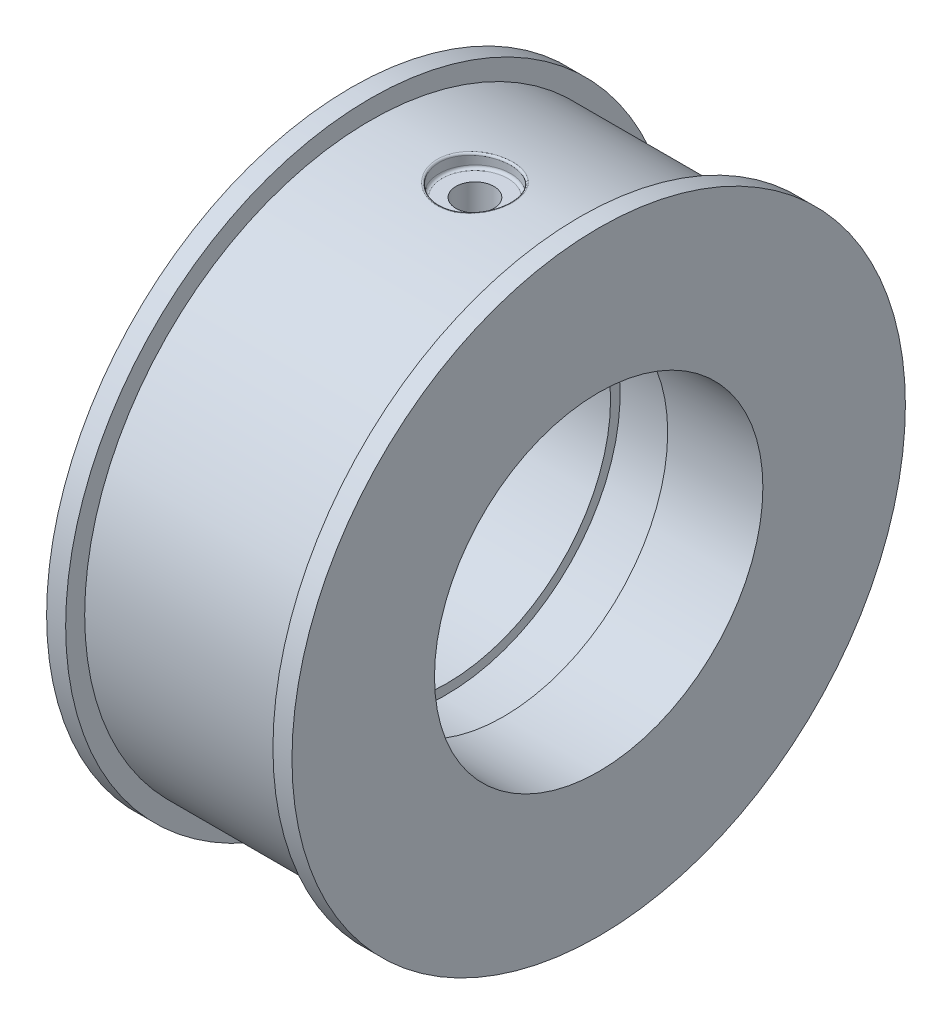
SolidWorks part; units mm, degrees
ref_plane "Front Plane" through (0, 0, 0) normal (0, 0, 1) x (1, 0, 0)
ref_plane "Top Plane" through (0, 0, 0) normal (0, 1, 0) x (1, 0, 0)
ref_plane "Right Plane" through (0, 0, 0) normal (1, 0, 0) x (0, 0, -1)
sketch "Sketch1" plane through (0, 0, 0) normal (0, 0, 1) x (1, 0, 0)
  line L0 (-19.0368, 0) -> (19.2228, 0) construction
  line L1 (-8.3897, 17.25) -> (-8.3897, 32)
  line L2 (-8.3897, 32) -> (-6.3897, 32)
  line L3 (-6.3897, 32) -> (-6.3897, 30)
  line L4 (-6.3897, 30) -> (15.6103, 30)
  line L5 (15.6103, 30) -> (15.6103, 32.223)
  line L6 (15.6103, 32.223) -> (17.6103, 32.223)
  line L7 (17.6103, 32.223) -> (17.6103, 17.25)
  line L8 (17.6103, 17.25) -> (7.6103, 17.25)
  line L9 (7.6103, 17.25) -> (7.6103, 18.25)
  line L10 (7.6103, 18.25) -> (1.6103, 18.25)
  line L11 (1.6103, 18.25) -> (1.6103, 17.25)
  line L12 (1.6103, 17.25) -> (-8.3897, 17.25)
  dimension "D2" = 26
  dimension "D3" = 22
  dimension "D4" = 2
  dimension "D5" = 17.25
  dimension "D6" = 17.25
  dimension "D7" = 18.25
  dimension "D8" = 6
  dimension "D9" = 10
  dimension "D10" = 30
revolve "Revolve1" add sketch "Sketch1" angle 360 about L0
ref_plane "Plane1" through (0, 30, 0) normal (0, 1, 0) x (1, 0, 0)
sketch "Sketch2" plane through (0, 30, 0) normal (0, 1, 0) x (1, 0, 0)
  line L0 (-6.3897, 0) -> (15.6103, 0)
  line L1 (-6.3897, -32) -> (-6.3897, 32) construction
  line L2 (15.6103, 30) -> (15.6103, -30) construction
hole_wizard "Hole1" positions "Sketch3" profile "Sketch4" legacy
sketch "Sketch3" plane through (0, 30, 0) normal (0, 1, 0) x (1, 0, 0)
  line L0 (-6.3897, 0) -> (15.6103, 0) construction
  point P0 (4.6103, 0)
sketch "Sketch4" plane through (4.6103, 30, 0) normal (1, 0, 0) x (0, 0, 1)
  line L0 (0, 0) -> (0, 1.5)
  line L1 (0, 1.5) -> (3.75, 1.5)
  line L2 (3.75, 1.5) -> (3.75, 0)
  line L3 (3.75, 0) -> (0, 0)
  line L4 (0, 110) -> (0, -10) construction
  dimension "直径" = 7.5
  dimension "深度" = 1.5
hole_wizard "Hole2" positions "Sketch5" profile "Sketch6" legacy
sketch "Sketch5" plane through (0, 28.5, 0) normal (0, 1, 0) x (1, 0, 0)
  point P0 (4.6103, 0)
sketch "Sketch6" plane through (4.6103, 28.5, 0) normal (1, 0, 0) x (0, 0, 1)
  line L0 (0, 0) -> (0, 10.25)
  line L1 (0, 10.25) -> (2, 10.25)
  line L2 (2, 10.25) -> (2, 0)
  line L3 (2, 0) -> (0, 0)
  line L4 (0, 110) -> (0, -10) construction
  dimension "直径" = 4
  dimension "深度" = 10.25
ref_plane "Plane2" through (0, -30, 0) normal (0, -1, 0) x (-1, 0, 0)
sketch "Sketch8" plane through (0, -30, 0) normal (0, -1, 0) x (-1, 0, 0)
  line L0 (6.3897, 0) -> (-15.6103, 0) construction
  line L1 (6.3897, 0) -> (-15.6103, 0)
hole_wizard "Dowel Hole1" positions "Sketch9" profile "Sketch10" hole size "Ø4.0" standard "GB"
sketch "Sketch9" plane through (0, -30, 0) normal (0, -1, 0) x (-1, 0, 0)
  line L0 (6.3897, 0) -> (-15.6103, 0) construction
  point P0 (-4.6103, 0)
sketch "Sketch10" plane through (4.6103, -30, 0) normal (1, 0, 0) x (0, 0, -1)
  line L0 (0, 0) -> (0, 5.2017)
  line L1 (0, 5.2017) -> (2, 4)
  line L2 (2, 4) -> (2, 0)
  line L5 (2, 0) -> (0, 0)
  line L10 (0, 5.2017) -> (-2, 4) construction
  line L11 (0, -6.35) -> (0, 107.95) construction
  dimension "孔直径" = 4
  dimension "孔深度" = 4
  dimension "导头角度" = 118
fillet "Fillet1" radius 0.2 1 edges at (5.44, 29.7763, -3.6571)
fillet "Fillet2" radius 0.3 1 edges at (4.6103, 28.5, 3.75)
